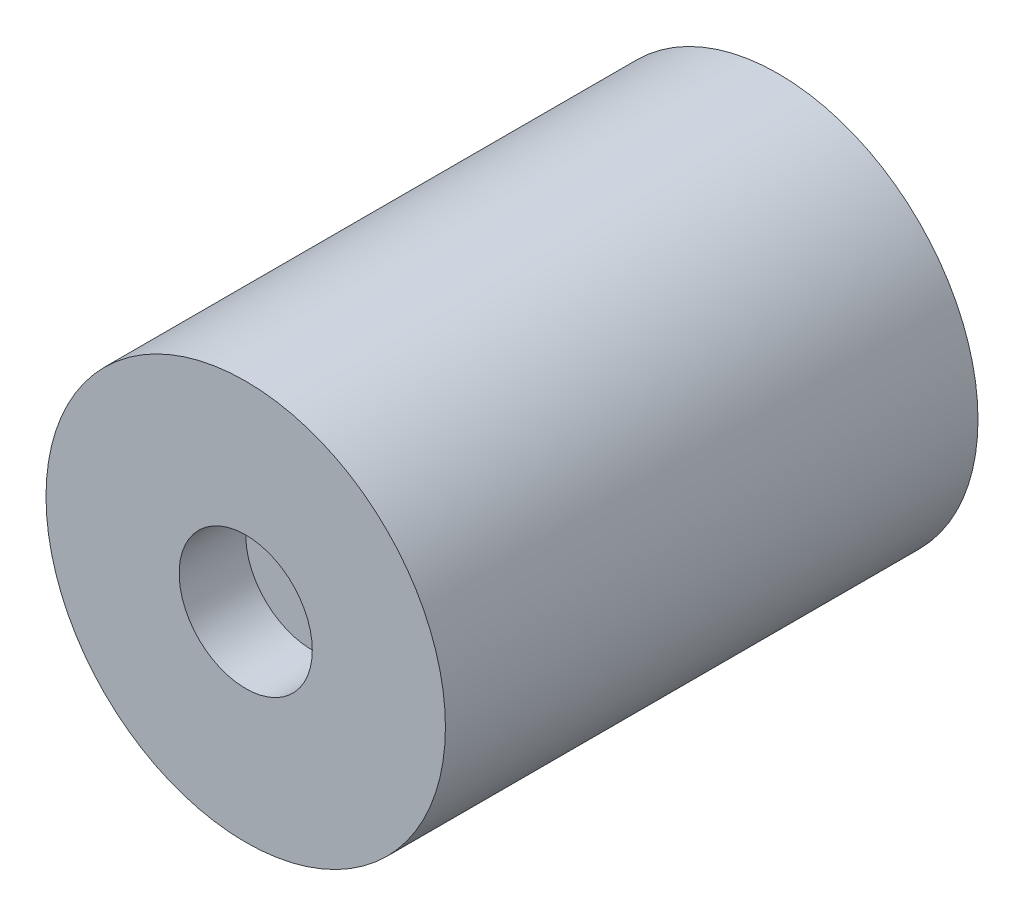
from build123d import *

# Parameters (mm, degrees)
SKETCH1_R           = 1.5
BOSS_EXTRUDE1_DEPTH = 4
SKETCH4_R           = 0.5
CUT_EXTRUDE1_DEPTH  = 0.5
CUT_EXTRUDE2_START  = -0.25
SKETCH5_R           = 0.5
CUT_EXTRUDE2_DEPTH  = 0.25


with BuildPart() as part:
    # Sketch1 → Boss-Extrude1 (new body)
    with BuildSketch(Plane.XY):
        with Locations((-276.531304302, -10.117720272)):
            Circle(SKETCH1_R)
    extrude(amount=BOSS_EXTRUDE1_DEPTH)

    # Sketch4 → Cut-Extrude1 (cut)
    with BuildSketch(Plane.XY.offset(4)):
        with Locations((-276.531304302, -10.117720272)):
            Circle(SKETCH4_R)
    extrude(amount=-CUT_EXTRUDE1_DEPTH, mode=Mode.SUBTRACT)

    # Sketch5 → Cut-Extrude2 (cut)
    with BuildSketch(Plane(origin=(0, 0, 0), x_dir=(-1, 0, 0), z_dir=(0, 0, -1)).offset(CUT_EXTRUDE2_START)):
        with Locations(Location((276.531304302, -10.117720272, 0), (0, 0, 180))):
            Circle(SKETCH5_R)
    extrude(amount=CUT_EXTRUDE2_DEPTH, mode=Mode.SUBTRACT)


solid = part.part
